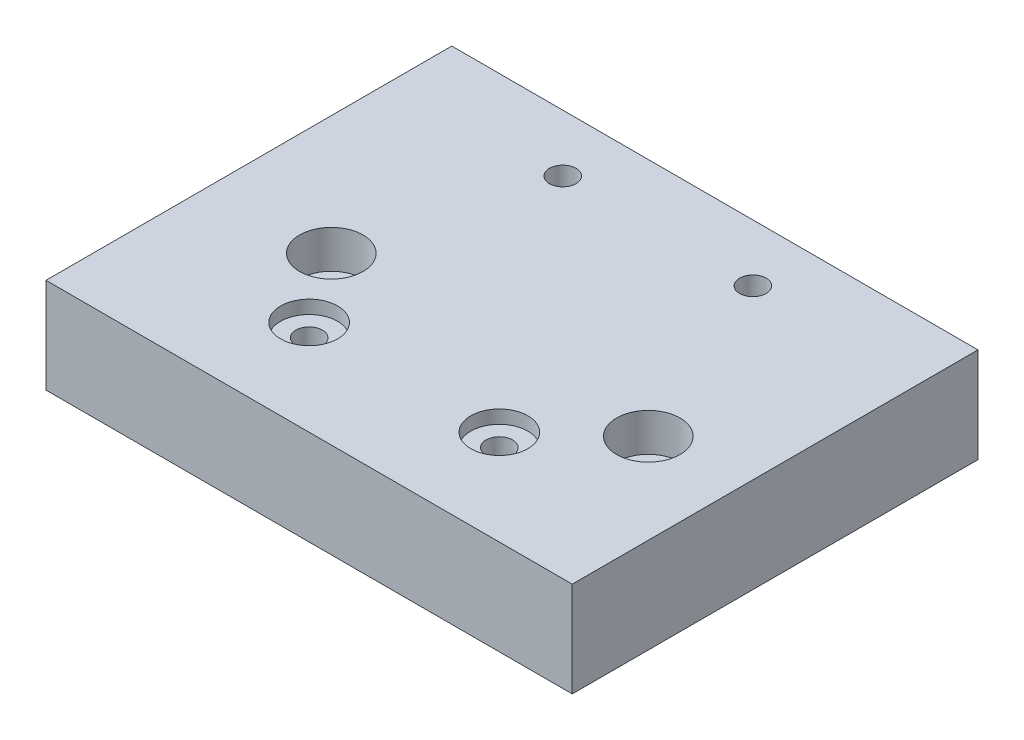
SolidWorks part; units mm, degrees
material "45"
ref_plane "Front Plane" through (0, 0, 0) normal (0, 0, 1) x (1, 0, 0)
ref_plane "Top Plane" through (0, 0, 0) normal (0, 1, 0) x (1, 0, 0)
ref_plane "Right Plane" through (0, 0, 0) normal (1, 0, 0) x (0, 0, -1)
sketch "Sketch1" plane through (0, 0, 0) normal (0, 0, 1) x (1, 0, 0)
  line L1 (0, 0) -> (83, 0)
  line L2 (0, 0) -> (0, 15)
  line L3 (0, 15) -> (83, 15)
  line L4 (83, 0) -> (83, 15)
  dimension "D1" = 15
  dimension "D2" = 83
extrude "Boss-Extrude1" add sketch "Sketch1" along normal blind 64
hole_wizard "Hole size per socket head cap screw type 1" positions "Sketch3" profile "Sketch4" counterbore size "M5" standard "Gb" end condition through all
sketch "Sketch3" plane through (0, 15, 0) normal (0, 1, 0) x (1, 0, 0)
  point P0 (18.8, -37.8)
  point P3 (68.8, -37.8)
sketch "Sketch4" plane through (18.8, 15, 37.8) normal (1, 0, 0) x (0, 0, 1)
  line L0 (0, 0) -> (0, 15)
  line L1 (0, 15) -> (2.75, 15)
  line L3 (2.75, 15) -> (2.75, 6)
  line L4 (2.75, 6) -> (5, 6)
  line L5 (5, 6) -> (5, 0)
  line L7 (5, 0) -> (0, 0)
  line L11 (0, -6.35) -> (0, 107.95) construction
  dimension "通孔孔直径" = 5.5
  dimension "通孔孔深度" = 15
  dimension "柱形沉头孔直径" = 10
  dimension "柱形沉头孔深度" = 6
sketch "Sketch5" plane through (0, 0, 0) normal (0, -1, 0) x (1, 0, 0)
  circle A0 centre (18.8, 37.8) radius 3.5
  circle A1 centre (68.8, 37.8) radius 3.5
  dimension "D1" = 7
extrude "Cut-Extrude1" cut sketch "Sketch5" against normal blind 1.6
hole_wizard "M5 Tapped Hole1" positions "Sketch7" profile "Sketch6" tap size "M5" standard "Iso" end condition through all
sketch "Sketch7" plane through (0, 15, 0) normal (0, 1, 0) x (1, 0, 0)
  point P0 (56.5, -9)
  point P3 (26.5, -9)
  point P6 (26.5, -49)
  point P9 (56.5, -49)
sketch "Sketch6" plane through (56.5, 15, 9) normal (1, 0, 0) x (0, 0, 1)
  line L0 (0, 0) -> (0, 15)
  line L1 (0, 15) -> (2.1, 15)
  line L2 (2.1, 15) -> (2.1, 0)
  line L5 (2.1, 0) -> (0, 0)
  line L11 (0, -6.35) -> (0, 107.95) construction
  dimension "通孔螺纹孔钻头直径" = 4.2
  dimension "通孔螺纹孔钻头深度" = 15
cosmetic thread "Hole thread 1" parameters "D2"=5
cosmetic thread "Hole thread 2" parameters "D2"=5
cosmetic thread "Hole thread 3" parameters "D2"=5
cosmetic thread "Hole thread 4" parameters "D2"=5
sketch "Sketch8" plane through (0, 15, 0) normal (0, 1, 0) x (1, 0, 0)
  circle A0 centre (26.5, -49) radius 4.5
  circle A1 centre (56.5, -49) radius 4.5
  dimension "D1" = 9
extrude "Cut-Extrude2" cut sketch "Sketch8" against normal blind 2.1
